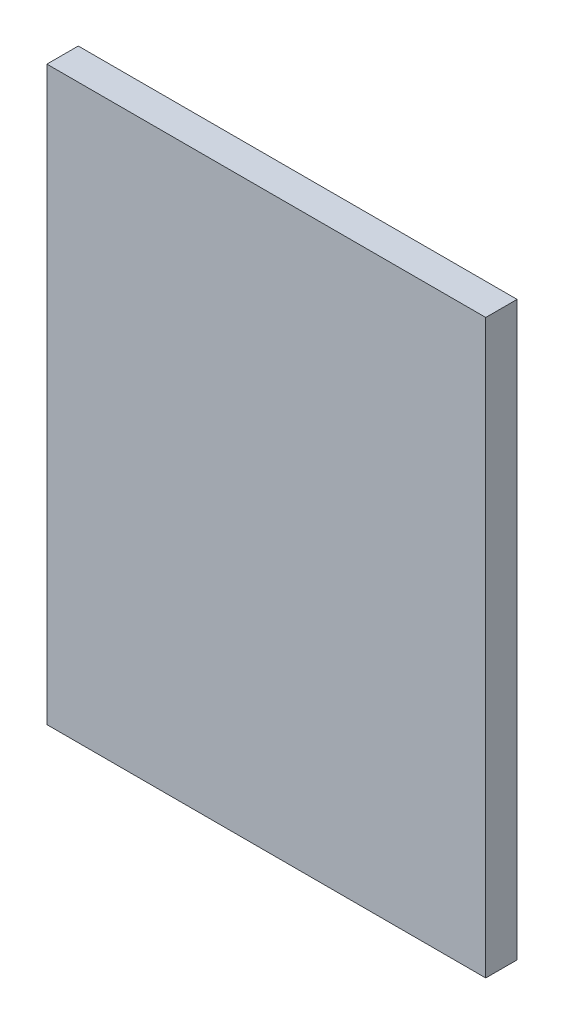
SolidWorks part; units mm, degrees
ref_plane "Front Plane" through (0, 0, 0) normal (0, 0, 1) x (1, 0, 0)
ref_plane "Top Plane" through (0, 0, 0) normal (0, 1, 0) x (1, 0, 0)
ref_plane "Right Plane" through (0, 0, 0) normal (1, 0, 0) x (0, 0, -1)
sketch "Sketch1" plane through (0, 0, 0) normal (0, 0, 1) x (1, 0, 0)
  line L1 (0, 0) -> (-280, 0)
  line L2 (0, 0) -> (0, 365)
  line L3 (0, 365) -> (-280, 365)
  line L4 (-280, 0) -> (-280, 365)
  dimension "D1" = 280
  dimension "D2" = 365
extrude "Boss-Extrude1" add sketch "Sketch1" along normal blind 20
